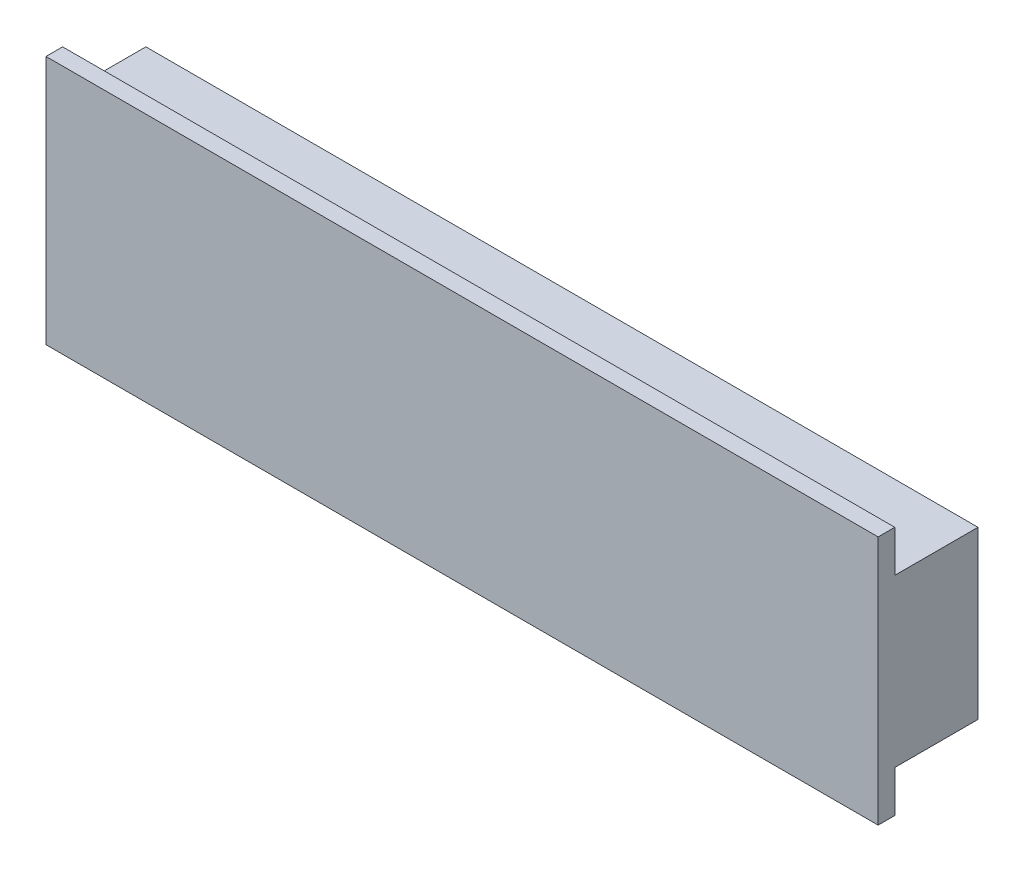
SolidWorks part; units mm, degrees
ref_plane "Front Plane" through (0, 0, 0) normal (0, 0, 1) x (1, 0, 0)
ref_plane "Top Plane" through (0, 0, 0) normal (0, 1, 0) x (1, 0, 0)
ref_plane "Right Plane" through (0, 0, 0) normal (1, 0, 0) x (0, 0, -1)
other "Configuration Table"
sketch "Sketch1" plane through (0, 0, 0) normal (0, 0, 1) x (1, 0, 0)
  line L1 (-250, 75) -> (250, 75)
  line L2 (-250, 75) -> (-250, -75)
  line L3 (-250, -75) -> (250, -75)
  line L4 (250, 75) -> (250, -75)
  line L5 (-250, 75) -> (250, -75) construction
  line L6 (-250, -75) -> (250, 75) construction
  point P0 (0, 0)
  dimension "D1" = 500
  dimension "D2" = 150
extrude "Boss-Extrude1" add sketch "Sketch1" along normal blind 10
sketch "Sketch2" plane through (0, 0, 0) normal (0, 0, -1) x (-1, 0, 0)
  line L0 (250, 75) -> (250, -75) construction
  line L1 (-250, 50) -> (250, 50)
  line L2 (-250, 50) -> (-250, -50)
  line L3 (-250, -50) -> (250, -50)
  line L4 (250, 50) -> (250, -50)
  line L5 (-250, 50) -> (250, -50) construction
  line L6 (-250, -50) -> (250, 50) construction
  point P0 (0, 0)
  dimension "D1" = 100
extrude "Boss-Extrude2" add sketch "Sketch2" along normal blind 50
